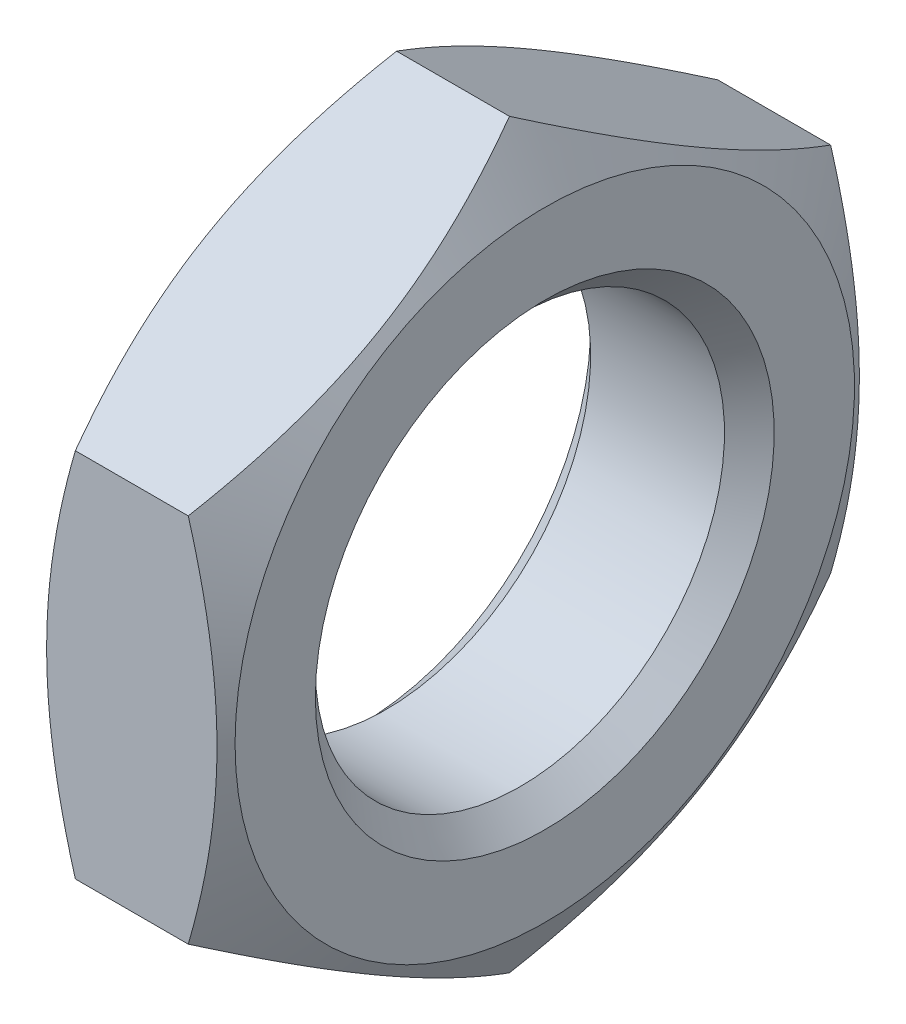
from build123d import *

# Parameters (mm, degrees)
BOSS_EXTRUDE1_DEPTH      = 2
BOSS_EXTRUDE1_DEPTH_BACK = 2


with BuildPart() as part:
    # Sketch1 → Boss-Extrude1 (new, two sides: drawn at the far end of the back side and taken through both)
    with BuildSketch(Plane(origin=(0, 0, 0), x_dir=(0, 0, -1), z_dir=(1, 0, 0)).offset(-BOSS_EXTRUDE1_DEPTH_BACK)):
        Polygon((-7, 4.041451884), (-7, -4.041451884), (0, -8.082903769), (7, -4.041451884), (7, 4.041451884), (0, 8.082903769), align=None)
    extrude(amount=BOSS_EXTRUDE1_DEPTH + BOSS_EXTRUDE1_DEPTH_BACK)

    # Sketch2 → Cut-Revolve1 (revolve, cut)
    with BuildSketch(Plane.XY, mode=Mode.PRIVATE) as cut_revolve1_sk:
        Polygon((-2, 0), (-2, 5), (-1.4585, 4.4585), (1.4585, 4.4585), (2, 5), (2, 0), align=None)
    revolve(cut_revolve1_sk.sketch.rotate(Axis((2, 0, 0), (-1, 0, 0)), 270), axis=Axis((2, 0, 0), (-1, 0, 0)), mode=Mode.SUBTRACT)

    # Sketch3 → Cut-Revolve2 (revolve, cut)
    with BuildSketch(Plane.XY, mode=Mode.PRIVATE) as cut_revolve2_sk:
        Polygon((-7, 16.75), (-7, 1), (-2, 1), (-2, 6.75), (0, 10.214101615), (2, 6.75), (2, 1), (7, 1), (7, 16.75), align=None)
    revolve(cut_revolve2_sk.sketch.rotate(Axis((50, 0, 0), (-1, 0, 0)), 270), axis=Axis((50, 0, 0), (-1, 0, 0)), mode=Mode.SUBTRACT)


solid = part.part
